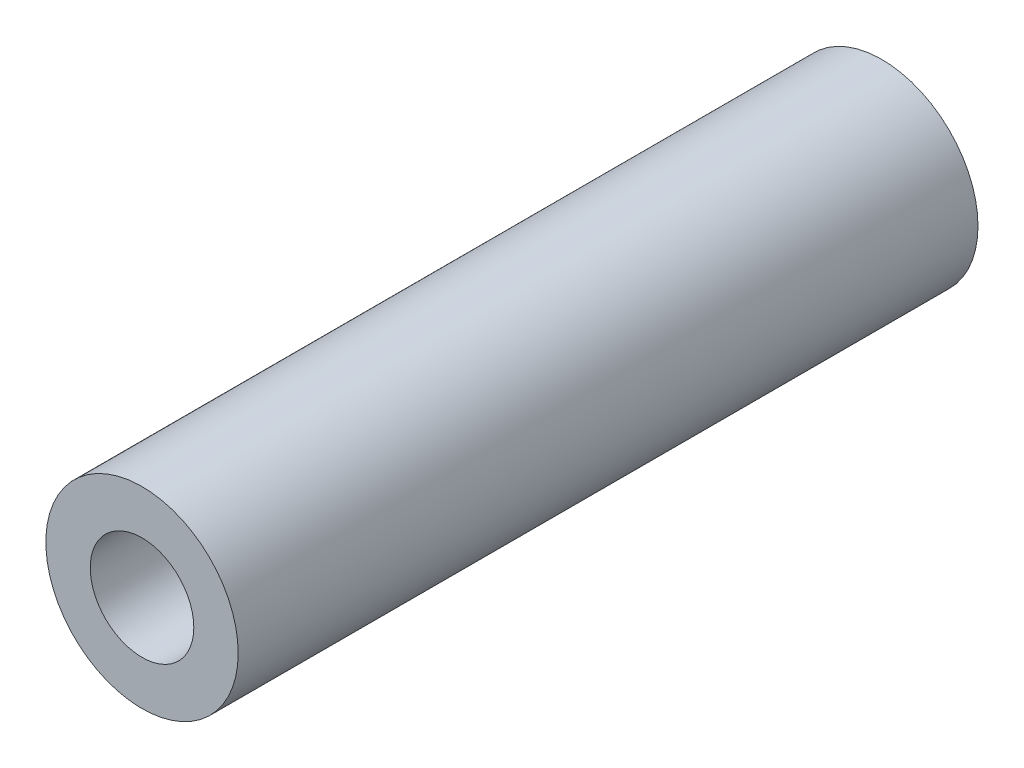
from build123d import *

# Parameters (mm, degrees)
SKETCH_1_R      = 6.5
SKETCH_1_R_2    = 3.5
EXTRUDE_1_DEPTH = 50


with BuildPart() as part:
    # 草图1 → 凸台-拉伸1 (new body)
    with BuildSketch(Plane.XY):
        Circle(SKETCH_1_R)
        Circle(SKETCH_1_R_2, mode=Mode.SUBTRACT)
    extrude(amount=EXTRUDE_1_DEPTH)


solid = part.part
